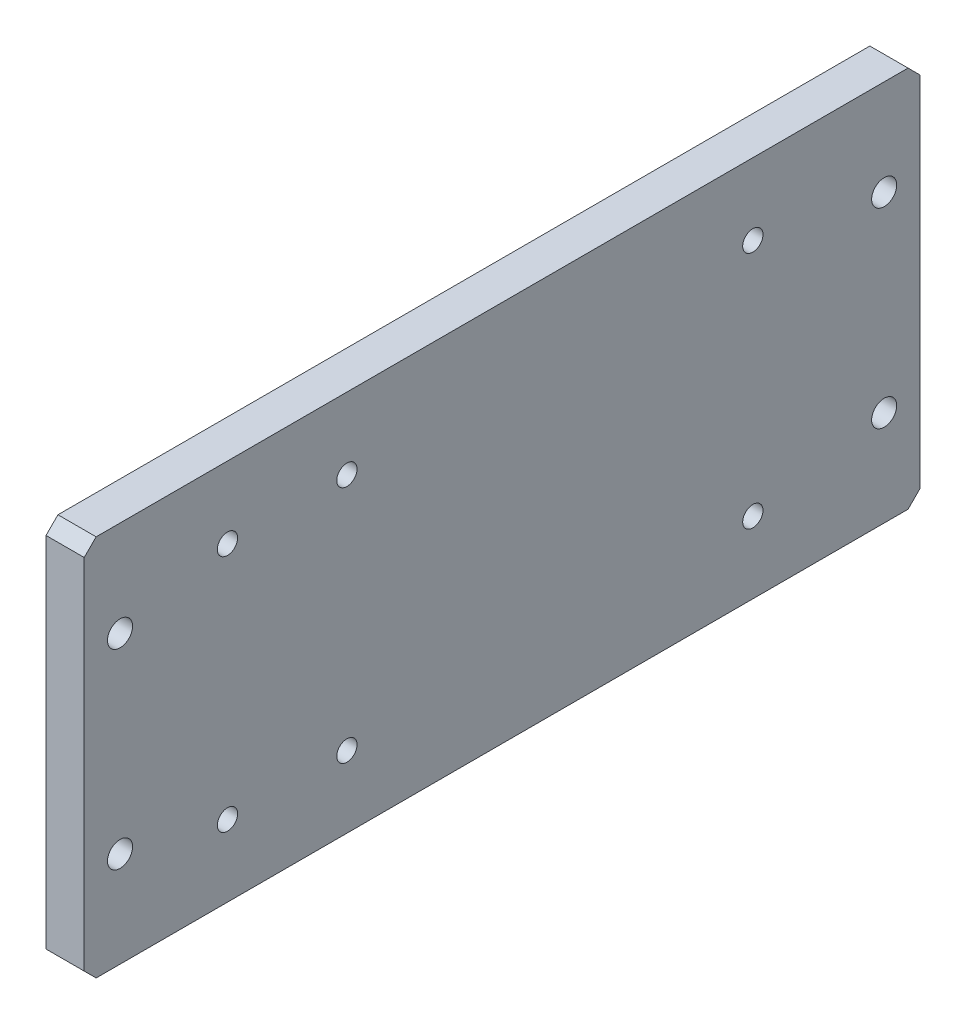
SolidWorks part; units mm, degrees
ref_plane "前视基准面" through (0, 0, 0) normal (0, 0, 1) x (1, 0, 0)
ref_plane "上视基准面" through (0, 0, 0) normal (0, 1, 0) x (1, 0, 0)
ref_plane "右视基准面" through (0, 0, 0) normal (1, 0, 0) x (0, 0, -1)
sketch "草图1" plane through (0, 0, 0) normal (1, 0, 0) x (0, 0, -1)
  line L1 (-175, 80) -> (175, 80)
  line L2 (-175, 80) -> (-175, -80)
  line L3 (-175, -80) -> (175, -80)
  line L4 (175, 80) -> (175, -80)
  line L5 (-175, 80) -> (175, -80) construction
  line L6 (-175, -80) -> (175, 80) construction
  point P0 (0, 0)
  dimension "D1" = 350
  dimension "D2" = 160
extrude "凸台-拉伸1" add sketch "草图1" along normal blind 16
hole_wizard "M10 螺纹孔1" positions "草图2" profile "草图3" tap size "M10" standard "GB" end condition through all
sketch "草图2" plane through (16, 0, 0) normal (1, 0, 0) x (0, 0, -1)
  line L0 (0, 0) -> (0, 50.2909) construction
  line L2 (0, 0) -> (64.5163, 0) construction
  point P0 (-115, 50)
  point P2 (-115, -50)
  point P4 (105, 50)
  point P6 (105, -50)
  point P17 (-65, 50)
  point P19 (-65, -50)
  dimension "D1" = 220
  dimension "D2" = 100
  dimension "D3" = 50
  dimension "D4" = 115
sketch "草图3" plane through (16, 50, 115) normal (0, 1, 0) x (0, 0, -1)
  line L0 (0, 0) -> (0, 16)
  line L1 (0, 16) -> (4.25, 16)
  line L2 (4.25, 16) -> (4.25, 0)
  line L5 (4.25, 0) -> (0, 0)
  line L11 (0, -6.35) -> (0, 107.95) construction
  dimension "通孔螺纹孔钻头直径" = 8.5
  dimension "通孔螺纹孔钻头深度" = 16
cosmetic thread "孔螺蚊线1" parameters "D2"=10
cosmetic thread "孔螺蚊线2" parameters "D2"=10
cosmetic thread "孔螺蚊线3" parameters "D2"=10
cosmetic thread "孔螺蚊线4" parameters "D2"=10
cosmetic thread "孔螺蚊线5" parameters "D2"=10
cosmetic thread "孔螺蚊线6" parameters "D2"=10
hole_wizard "Ø10.5 (10.5) 直径孔1" positions "草图4" profile "草图5" hole size "Ø10.5" standard "GB" end condition through all
sketch "草图4" plane through (0, 0, 0) normal (-1, 0, 0) x (0, 0, 1)
  line L0 (0, 46.8735) -> (0, 0) construction
  line L1 (0, 0) -> (94.5904, 0) construction
  point P0 (-160, 40)
  point P2 (-160, -40)
  point P4 (160, 40)
  point P6 (160, -40)
  dimension "D1" = 320
  dimension "D2" = 80
sketch "草图5" plane through (0, 40, -160) normal (0, 1, 0) x (0, 0, 1)
  line L0 (0, 0) -> (0, 16)
  line L1 (0, 16) -> (5.25, 16)
  line L2 (5.25, 16) -> (5.25, 0)
  line L5 (5.25, 0) -> (0, 0)
  line L11 (0, -6.35) -> (0, 107.95) construction
  dimension "通孔孔直径" = 10.5
  dimension "通孔孔深度" = 16
chamfer "倒角1" distance 5 angle 45 4 edges at (8, 80, 175) (8, -80, 175) (8, 80, -175) (8, -80, -175)
